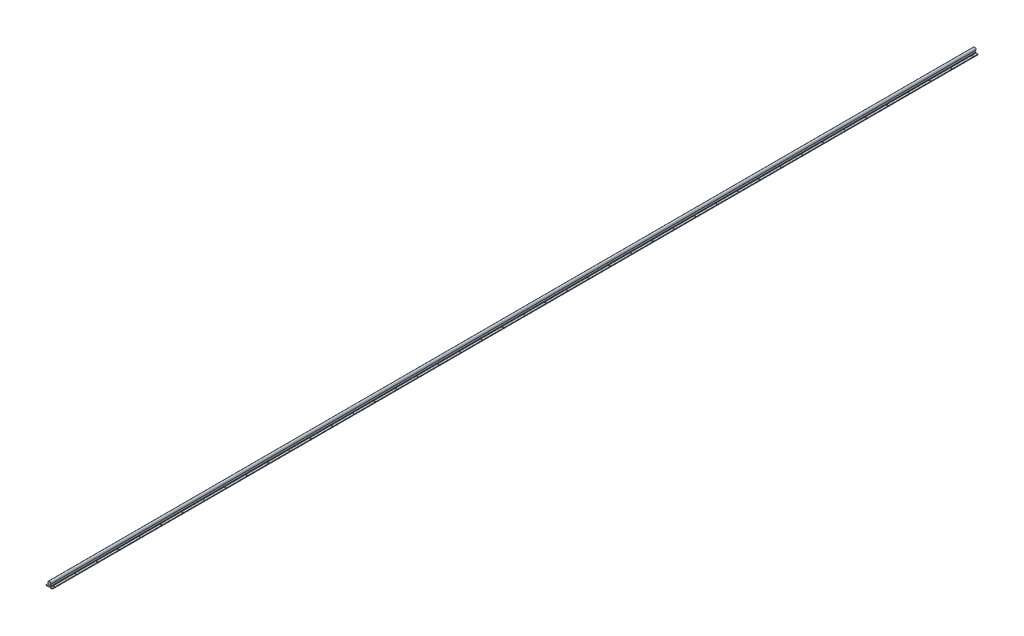
from build123d import *

# Parameters (mm, degrees)
BOSS_EXTRUDE1_DEPTH        = 6500
SKETCH5_R                  = 2.75
CUT_EXTRUDE1_DEPTH         = 6501.117710473
LPATTERN1_COUNT            = 44
LPATTERN1_PITCH            = 150
LPATTERN1_COPY_1_SKETCH_R  = 2.75
LPATTERN1_COPY_1_DEPTH     = 6501.117710473
LPATTERN1_COPY_2_SKETCH_R  = 2.75
LPATTERN1_COPY_2_DEPTH     = 6501.117710473
LPATTERN1_COPY_3_SKETCH_R  = 2.75
LPATTERN1_COPY_3_DEPTH     = 6501.117710473
LPATTERN1_COPY_4_SKETCH_R  = 2.75
LPATTERN1_COPY_4_DEPTH     = 6501.117710473
LPATTERN1_COPY_5_SKETCH_R  = 2.75
LPATTERN1_COPY_5_DEPTH     = 6501.117710473
LPATTERN1_COPY_6_SKETCH_R  = 2.75
LPATTERN1_COPY_6_DEPTH     = 6501.117710473
LPATTERN1_COPY_7_SKETCH_R  = 2.75
LPATTERN1_COPY_7_DEPTH     = 6501.117710473
LPATTERN1_COPY_8_SKETCH_R  = 2.75
LPATTERN1_COPY_8_DEPTH     = 6501.117710473
LPATTERN1_COPY_9_SKETCH_R  = 2.75
LPATTERN1_COPY_9_DEPTH     = 6501.117710473
LPATTERN1_COPY_10_SKETCH_R = 2.75
LPATTERN1_COPY_10_DEPTH    = 6501.117710473
LPATTERN1_COPY_11_SKETCH_R = 2.75
LPATTERN1_COPY_11_DEPTH    = 6501.117710473
LPATTERN1_COPY_12_SKETCH_R = 2.75
LPATTERN1_COPY_12_DEPTH    = 6501.117710473
LPATTERN1_COPY_13_SKETCH_R = 2.75
LPATTERN1_COPY_13_DEPTH    = 6501.117710473
LPATTERN1_COPY_14_SKETCH_R = 2.75
LPATTERN1_COPY_14_DEPTH    = 6501.117710473
LPATTERN1_COPY_15_SKETCH_R = 2.75
LPATTERN1_COPY_15_DEPTH    = 6501.117710473
LPATTERN1_COPY_16_SKETCH_R = 2.75
LPATTERN1_COPY_16_DEPTH    = 6501.117710473
LPATTERN1_COPY_17_SKETCH_R = 2.75
LPATTERN1_COPY_17_DEPTH    = 6501.117710473
LPATTERN1_COPY_18_SKETCH_R = 2.75
LPATTERN1_COPY_18_DEPTH    = 6501.117710473
LPATTERN1_COPY_19_SKETCH_R = 2.75
LPATTERN1_COPY_19_DEPTH    = 6501.117710473
LPATTERN1_COPY_20_SKETCH_R = 2.75
LPATTERN1_COPY_20_DEPTH    = 6501.117710473
LPATTERN1_COPY_21_SKETCH_R = 2.75
LPATTERN1_COPY_21_DEPTH    = 6501.117710473
LPATTERN1_COPY_22_SKETCH_R = 2.75
LPATTERN1_COPY_22_DEPTH    = 6501.117710473
LPATTERN1_COPY_23_SKETCH_R = 2.75
LPATTERN1_COPY_23_DEPTH    = 6501.117710473
LPATTERN1_COPY_24_SKETCH_R = 2.75
LPATTERN1_COPY_24_DEPTH    = 6501.117710473
LPATTERN1_COPY_25_SKETCH_R = 2.75
LPATTERN1_COPY_25_DEPTH    = 6501.117710473
LPATTERN1_COPY_26_SKETCH_R = 2.75
LPATTERN1_COPY_26_DEPTH    = 6501.117710473
LPATTERN1_COPY_27_SKETCH_R = 2.75
LPATTERN1_COPY_27_DEPTH    = 6501.117710473
LPATTERN1_COPY_28_SKETCH_R = 2.75
LPATTERN1_COPY_28_DEPTH    = 6501.117710473
LPATTERN1_COPY_29_SKETCH_R = 2.75
LPATTERN1_COPY_29_DEPTH    = 6501.117710473
LPATTERN1_COPY_30_SKETCH_R = 2.75
LPATTERN1_COPY_30_DEPTH    = 6501.117710473
LPATTERN1_COPY_31_SKETCH_R = 2.75
LPATTERN1_COPY_31_DEPTH    = 6501.117710473
LPATTERN1_COPY_32_SKETCH_R = 2.75
LPATTERN1_COPY_32_DEPTH    = 6501.117710473
LPATTERN1_COPY_33_SKETCH_R = 2.75
LPATTERN1_COPY_33_DEPTH    = 6501.117710473
LPATTERN1_COPY_34_SKETCH_R = 2.75
LPATTERN1_COPY_34_DEPTH    = 6501.117710473
LPATTERN1_COPY_35_SKETCH_R = 2.75
LPATTERN1_COPY_35_DEPTH    = 6501.117710473
LPATTERN1_COPY_36_SKETCH_R = 2.75
LPATTERN1_COPY_36_DEPTH    = 6501.117710473
LPATTERN1_COPY_37_SKETCH_R = 2.75
LPATTERN1_COPY_37_DEPTH    = 6501.117710473
LPATTERN1_COPY_38_SKETCH_R = 2.75
LPATTERN1_COPY_38_DEPTH    = 6501.117710473
LPATTERN1_COPY_39_SKETCH_R = 2.75
LPATTERN1_COPY_39_DEPTH    = 6501.117710473
LPATTERN1_COPY_40_SKETCH_R = 2.75
LPATTERN1_COPY_40_DEPTH    = 6501.117710473
LPATTERN1_COPY_41_SKETCH_R = 2.75
LPATTERN1_COPY_41_DEPTH    = 6501.117710473
LPATTERN1_COPY_42_SKETCH_R = 2.75
LPATTERN1_COPY_42_DEPTH    = 6501.117710473
LPATTERN1_COPY_43_SKETCH_R = 2.75
LPATTERN1_COPY_43_DEPTH    = 6501.117710473
CHAMFER1_SIZE              = 1


with BuildPart() as part:
    # Sketch3 → Boss-Extrude1 (new body)
    with BuildSketch(Plane.XY):
        with BuildLine():
            Line((-5.5, -20.5), (5.5, -20.5))
            Line((5.5, -20.5), (5.5, -27))
            Line((5.5, -27), (22.5, -27))
            Line((22.5, -27), (22.5, -22))
            Line((22.5, -22), (9.5, -22))
            Line((9.5, -22), (9.5, -17))
            Line((9.5, -17), (8.445597073, -17))
            Line((8.445597073, -17), (4, -9.3))
            Line((4, -9.3), (4, -9.16515139))
            ThreePointArc((4, -9.16515139), (0, 10), (-4, -9.16515139))
            Line((-4, -9.16515139), (-4, -9.3))
            Line((-4, -9.3), (-8.445597073, -17))
            Line((-8.445597073, -17), (-9.5, -17))
            Line((-9.5, -17), (-9.5, -22))
            Line((-9.5, -22), (-22.5, -22))
            Line((-22.5, -22), (-22.5, -27))
            Line((-22.5, -27), (-5.5, -27))
            Line((-5.5, -27), (-5.5, -20.5))
        make_face()
    extrude(amount=-BOSS_EXTRUDE1_DEPTH)

    # Sketch4 → Cut-Revolve1 (revolve, cut)
    with BuildSketch(Plane(origin=(0, 0, 0), x_dir=(0, 0, -1), z_dir=(1, 0, 0)), mode=Mode.PRIVATE) as cut_revolve1_sk:
        Polygon((22.805, 2.195), (20, 5), (20, -27), (23.3, -27), (23.3, -9.3), (22.805, -8.805), align=None)
    cut_revolve1 = revolve(cut_revolve1_sk.sketch.rotate(Axis((0, 5, -20), (0, -1, 0)), 180), axis=Axis((0, 5, -20), (0, -1, 0)), mode=Mode.SUBTRACT)

    # Sketch5 → Cut-Extrude1 (cut, through all)
    with BuildSketch(Plane(origin=(0, -22, 0), x_dir=(1, 0, 0), z_dir=(0, 1, 0))):
        with Locations(Location((15, 20, 0), (0, 0, 270))):
            Circle(SKETCH5_R)
    cut_extrude1 = extrude(amount=-CUT_EXTRUDE1_DEPTH, mode=Mode.SUBTRACT)

    # Mirror1: Cut-Extrude1 across plane
    add(cut_extrude1.mirror(Plane(origin=(0, 0, 0), x_dir=(0, 0, 1), z_dir=(1, 0, 0))), mode=Mode.SUBTRACT)

    # LPattern1: Cut-Revolve1, Cut-Extrude1 ×44
    with Locations(*[(0, 0, -i * LPATTERN1_PITCH) for i in range(1, LPATTERN1_COUNT)]):
        add(cut_revolve1, mode=Mode.SUBTRACT)
        add(cut_extrude1, mode=Mode.SUBTRACT)

    # LPattern1 copy 1 sketch → LPattern1 copy 1 (cut, through all)
    with BuildSketch(Plane(origin=(0, -22, -150), x_dir=(-1, 0, 0), z_dir=(0, 1, 0))):
        with Locations((15, -20)):
            Circle(LPATTERN1_COPY_1_SKETCH_R)
    extrude(amount=-LPATTERN1_COPY_1_DEPTH, mode=Mode.SUBTRACT)

    # LPattern1 copy 2 sketch → LPattern1 copy 2 (cut, through all)
    with BuildSketch(Plane(origin=(0, -22, -300), x_dir=(-1, 0, 0), z_dir=(0, 1, 0))):
        with Locations((15, -20)):
            Circle(LPATTERN1_COPY_2_SKETCH_R)
    extrude(amount=-LPATTERN1_COPY_2_DEPTH, mode=Mode.SUBTRACT)

    # LPattern1 copy 3 sketch → LPattern1 copy 3 (cut, through all)
    with BuildSketch(Plane(origin=(0, -22, -450), x_dir=(-1, 0, 0), z_dir=(0, 1, 0))):
        with Locations((15, -20)):
            Circle(LPATTERN1_COPY_3_SKETCH_R)
    extrude(amount=-LPATTERN1_COPY_3_DEPTH, mode=Mode.SUBTRACT)

    # LPattern1 copy 4 sketch → LPattern1 copy 4 (cut, through all)
    with BuildSketch(Plane(origin=(0, -22, -600), x_dir=(-1, 0, 0), z_dir=(0, 1, 0))):
        with Locations((15, -20)):
            Circle(LPATTERN1_COPY_4_SKETCH_R)
    extrude(amount=-LPATTERN1_COPY_4_DEPTH, mode=Mode.SUBTRACT)

    # LPattern1 copy 5 sketch → LPattern1 copy 5 (cut, through all)
    with BuildSketch(Plane(origin=(0, -22, -750), x_dir=(-1, 0, 0), z_dir=(0, 1, 0))):
        with Locations((15, -20)):
            Circle(LPATTERN1_COPY_5_SKETCH_R)
    extrude(amount=-LPATTERN1_COPY_5_DEPTH, mode=Mode.SUBTRACT)

    # LPattern1 copy 6 sketch → LPattern1 copy 6 (cut, through all)
    with BuildSketch(Plane(origin=(0, -22, -900), x_dir=(-1, 0, 0), z_dir=(0, 1, 0))):
        with Locations((15, -20)):
            Circle(LPATTERN1_COPY_6_SKETCH_R)
    extrude(amount=-LPATTERN1_COPY_6_DEPTH, mode=Mode.SUBTRACT)

    # LPattern1 copy 7 sketch → LPattern1 copy 7 (cut, through all)
    with BuildSketch(Plane(origin=(0, -22, -1050), x_dir=(-1, 0, 0), z_dir=(0, 1, 0))):
        with Locations((15, -20)):
            Circle(LPATTERN1_COPY_7_SKETCH_R)
    extrude(amount=-LPATTERN1_COPY_7_DEPTH, mode=Mode.SUBTRACT)

    # LPattern1 copy 8 sketch → LPattern1 copy 8 (cut, through all)
    with BuildSketch(Plane(origin=(0, -22, -1200), x_dir=(-1, 0, 0), z_dir=(0, 1, 0))):
        with Locations((15, -20)):
            Circle(LPATTERN1_COPY_8_SKETCH_R)
    extrude(amount=-LPATTERN1_COPY_8_DEPTH, mode=Mode.SUBTRACT)

    # LPattern1 copy 9 sketch → LPattern1 copy 9 (cut, through all)
    with BuildSketch(Plane(origin=(0, -22, -1350), x_dir=(-1, 0, 0), z_dir=(0, 1, 0))):
        with Locations((15, -20)):
            Circle(LPATTERN1_COPY_9_SKETCH_R)
    extrude(amount=-LPATTERN1_COPY_9_DEPTH, mode=Mode.SUBTRACT)

    # LPattern1 copy 10 sketch → LPattern1 copy 10 (cut, through all)
    with BuildSketch(Plane(origin=(0, -22, -1500), x_dir=(-1, 0, 0), z_dir=(0, 1, 0))):
        with Locations((15, -20)):
            Circle(LPATTERN1_COPY_10_SKETCH_R)
    extrude(amount=-LPATTERN1_COPY_10_DEPTH, mode=Mode.SUBTRACT)

    # LPattern1 copy 11 sketch → LPattern1 copy 11 (cut, through all)
    with BuildSketch(Plane(origin=(0, -22, -1650), x_dir=(-1, 0, 0), z_dir=(0, 1, 0))):
        with Locations((15, -20)):
            Circle(LPATTERN1_COPY_11_SKETCH_R)
    extrude(amount=-LPATTERN1_COPY_11_DEPTH, mode=Mode.SUBTRACT)

    # LPattern1 copy 12 sketch → LPattern1 copy 12 (cut, through all)
    with BuildSketch(Plane(origin=(0, -22, -1800), x_dir=(-1, 0, 0), z_dir=(0, 1, 0))):
        with Locations((15, -20)):
            Circle(LPATTERN1_COPY_12_SKETCH_R)
    extrude(amount=-LPATTERN1_COPY_12_DEPTH, mode=Mode.SUBTRACT)

    # LPattern1 copy 13 sketch → LPattern1 copy 13 (cut, through all)
    with BuildSketch(Plane(origin=(0, -22, -1950), x_dir=(-1, 0, 0), z_dir=(0, 1, 0))):
        with Locations((15, -20)):
            Circle(LPATTERN1_COPY_13_SKETCH_R)
    extrude(amount=-LPATTERN1_COPY_13_DEPTH, mode=Mode.SUBTRACT)

    # LPattern1 copy 14 sketch → LPattern1 copy 14 (cut, through all)
    with BuildSketch(Plane(origin=(0, -22, -2100), x_dir=(-1, 0, 0), z_dir=(0, 1, 0))):
        with Locations((15, -20)):
            Circle(LPATTERN1_COPY_14_SKETCH_R)
    extrude(amount=-LPATTERN1_COPY_14_DEPTH, mode=Mode.SUBTRACT)

    # LPattern1 copy 15 sketch → LPattern1 copy 15 (cut, through all)
    with BuildSketch(Plane(origin=(0, -22, -2250), x_dir=(-1, 0, 0), z_dir=(0, 1, 0))):
        with Locations((15, -20)):
            Circle(LPATTERN1_COPY_15_SKETCH_R)
    extrude(amount=-LPATTERN1_COPY_15_DEPTH, mode=Mode.SUBTRACT)

    # LPattern1 copy 16 sketch → LPattern1 copy 16 (cut, through all)
    with BuildSketch(Plane(origin=(0, -22, -2400), x_dir=(-1, 0, 0), z_dir=(0, 1, 0))):
        with Locations((15, -20)):
            Circle(LPATTERN1_COPY_16_SKETCH_R)
    extrude(amount=-LPATTERN1_COPY_16_DEPTH, mode=Mode.SUBTRACT)

    # LPattern1 copy 17 sketch → LPattern1 copy 17 (cut, through all)
    with BuildSketch(Plane(origin=(0, -22, -2550), x_dir=(-1, 0, 0), z_dir=(0, 1, 0))):
        with Locations((15, -20)):
            Circle(LPATTERN1_COPY_17_SKETCH_R)
    extrude(amount=-LPATTERN1_COPY_17_DEPTH, mode=Mode.SUBTRACT)

    # LPattern1 copy 18 sketch → LPattern1 copy 18 (cut, through all)
    with BuildSketch(Plane(origin=(0, -22, -2700), x_dir=(-1, 0, 0), z_dir=(0, 1, 0))):
        with Locations((15, -20)):
            Circle(LPATTERN1_COPY_18_SKETCH_R)
    extrude(amount=-LPATTERN1_COPY_18_DEPTH, mode=Mode.SUBTRACT)

    # LPattern1 copy 19 sketch → LPattern1 copy 19 (cut, through all)
    with BuildSketch(Plane(origin=(0, -22, -2850), x_dir=(-1, 0, 0), z_dir=(0, 1, 0))):
        with Locations((15, -20)):
            Circle(LPATTERN1_COPY_19_SKETCH_R)
    extrude(amount=-LPATTERN1_COPY_19_DEPTH, mode=Mode.SUBTRACT)

    # LPattern1 copy 20 sketch → LPattern1 copy 20 (cut, through all)
    with BuildSketch(Plane(origin=(0, -22, -3000), x_dir=(-1, 0, 0), z_dir=(0, 1, 0))):
        with Locations((15, -20)):
            Circle(LPATTERN1_COPY_20_SKETCH_R)
    extrude(amount=-LPATTERN1_COPY_20_DEPTH, mode=Mode.SUBTRACT)

    # LPattern1 copy 21 sketch → LPattern1 copy 21 (cut, through all)
    with BuildSketch(Plane(origin=(0, -22, -3150), x_dir=(-1, 0, 0), z_dir=(0, 1, 0))):
        with Locations((15, -20)):
            Circle(LPATTERN1_COPY_21_SKETCH_R)
    extrude(amount=-LPATTERN1_COPY_21_DEPTH, mode=Mode.SUBTRACT)

    # LPattern1 copy 22 sketch → LPattern1 copy 22 (cut, through all)
    with BuildSketch(Plane(origin=(0, -22, -3300), x_dir=(-1, 0, 0), z_dir=(0, 1, 0))):
        with Locations((15, -20)):
            Circle(LPATTERN1_COPY_22_SKETCH_R)
    extrude(amount=-LPATTERN1_COPY_22_DEPTH, mode=Mode.SUBTRACT)

    # LPattern1 copy 23 sketch → LPattern1 copy 23 (cut, through all)
    with BuildSketch(Plane(origin=(0, -22, -3450), x_dir=(-1, 0, 0), z_dir=(0, 1, 0))):
        with Locations((15, -20)):
            Circle(LPATTERN1_COPY_23_SKETCH_R)
    extrude(amount=-LPATTERN1_COPY_23_DEPTH, mode=Mode.SUBTRACT)

    # LPattern1 copy 24 sketch → LPattern1 copy 24 (cut, through all)
    with BuildSketch(Plane(origin=(0, -22, -3600), x_dir=(-1, 0, 0), z_dir=(0, 1, 0))):
        with Locations((15, -20)):
            Circle(LPATTERN1_COPY_24_SKETCH_R)
    extrude(amount=-LPATTERN1_COPY_24_DEPTH, mode=Mode.SUBTRACT)

    # LPattern1 copy 25 sketch → LPattern1 copy 25 (cut, through all)
    with BuildSketch(Plane(origin=(0, -22, -3750), x_dir=(-1, 0, 0), z_dir=(0, 1, 0))):
        with Locations((15, -20)):
            Circle(LPATTERN1_COPY_25_SKETCH_R)
    extrude(amount=-LPATTERN1_COPY_25_DEPTH, mode=Mode.SUBTRACT)

    # LPattern1 copy 26 sketch → LPattern1 copy 26 (cut, through all)
    with BuildSketch(Plane(origin=(0, -22, -3900), x_dir=(-1, 0, 0), z_dir=(0, 1, 0))):
        with Locations((15, -20)):
            Circle(LPATTERN1_COPY_26_SKETCH_R)
    extrude(amount=-LPATTERN1_COPY_26_DEPTH, mode=Mode.SUBTRACT)

    # LPattern1 copy 27 sketch → LPattern1 copy 27 (cut, through all)
    with BuildSketch(Plane(origin=(0, -22, -4050), x_dir=(-1, 0, 0), z_dir=(0, 1, 0))):
        with Locations((15, -20)):
            Circle(LPATTERN1_COPY_27_SKETCH_R)
    extrude(amount=-LPATTERN1_COPY_27_DEPTH, mode=Mode.SUBTRACT)

    # LPattern1 copy 28 sketch → LPattern1 copy 28 (cut, through all)
    with BuildSketch(Plane(origin=(0, -22, -4200), x_dir=(-1, 0, 0), z_dir=(0, 1, 0))):
        with Locations((15, -20)):
            Circle(LPATTERN1_COPY_28_SKETCH_R)
    extrude(amount=-LPATTERN1_COPY_28_DEPTH, mode=Mode.SUBTRACT)

    # LPattern1 copy 29 sketch → LPattern1 copy 29 (cut, through all)
    with BuildSketch(Plane(origin=(0, -22, -4350), x_dir=(-1, 0, 0), z_dir=(0, 1, 0))):
        with Locations((15, -20)):
            Circle(LPATTERN1_COPY_29_SKETCH_R)
    extrude(amount=-LPATTERN1_COPY_29_DEPTH, mode=Mode.SUBTRACT)

    # LPattern1 copy 30 sketch → LPattern1 copy 30 (cut, through all)
    with BuildSketch(Plane(origin=(0, -22, -4500), x_dir=(-1, 0, 0), z_dir=(0, 1, 0))):
        with Locations((15, -20)):
            Circle(LPATTERN1_COPY_30_SKETCH_R)
    extrude(amount=-LPATTERN1_COPY_30_DEPTH, mode=Mode.SUBTRACT)

    # LPattern1 copy 31 sketch → LPattern1 copy 31 (cut, through all)
    with BuildSketch(Plane(origin=(0, -22, -4650), x_dir=(-1, 0, 0), z_dir=(0, 1, 0))):
        with Locations((15, -20)):
            Circle(LPATTERN1_COPY_31_SKETCH_R)
    extrude(amount=-LPATTERN1_COPY_31_DEPTH, mode=Mode.SUBTRACT)

    # LPattern1 copy 32 sketch → LPattern1 copy 32 (cut, through all)
    with BuildSketch(Plane(origin=(0, -22, -4800), x_dir=(-1, 0, 0), z_dir=(0, 1, 0))):
        with Locations((15, -20)):
            Circle(LPATTERN1_COPY_32_SKETCH_R)
    extrude(amount=-LPATTERN1_COPY_32_DEPTH, mode=Mode.SUBTRACT)

    # LPattern1 copy 33 sketch → LPattern1 copy 33 (cut, through all)
    with BuildSketch(Plane(origin=(0, -22, -4950), x_dir=(-1, 0, 0), z_dir=(0, 1, 0))):
        with Locations((15, -20)):
            Circle(LPATTERN1_COPY_33_SKETCH_R)
    extrude(amount=-LPATTERN1_COPY_33_DEPTH, mode=Mode.SUBTRACT)

    # LPattern1 copy 34 sketch → LPattern1 copy 34 (cut, through all)
    with BuildSketch(Plane(origin=(0, -22, -5100), x_dir=(-1, 0, 0), z_dir=(0, 1, 0))):
        with Locations((15, -20)):
            Circle(LPATTERN1_COPY_34_SKETCH_R)
    extrude(amount=-LPATTERN1_COPY_34_DEPTH, mode=Mode.SUBTRACT)

    # LPattern1 copy 35 sketch → LPattern1 copy 35 (cut, through all)
    with BuildSketch(Plane(origin=(0, -22, -5250), x_dir=(-1, 0, 0), z_dir=(0, 1, 0))):
        with Locations((15, -20)):
            Circle(LPATTERN1_COPY_35_SKETCH_R)
    extrude(amount=-LPATTERN1_COPY_35_DEPTH, mode=Mode.SUBTRACT)

    # LPattern1 copy 36 sketch → LPattern1 copy 36 (cut, through all)
    with BuildSketch(Plane(origin=(0, -22, -5400), x_dir=(-1, 0, 0), z_dir=(0, 1, 0))):
        with Locations((15, -20)):
            Circle(LPATTERN1_COPY_36_SKETCH_R)
    extrude(amount=-LPATTERN1_COPY_36_DEPTH, mode=Mode.SUBTRACT)

    # LPattern1 copy 37 sketch → LPattern1 copy 37 (cut, through all)
    with BuildSketch(Plane(origin=(0, -22, -5550), x_dir=(-1, 0, 0), z_dir=(0, 1, 0))):
        with Locations((15, -20)):
            Circle(LPATTERN1_COPY_37_SKETCH_R)
    extrude(amount=-LPATTERN1_COPY_37_DEPTH, mode=Mode.SUBTRACT)

    # LPattern1 copy 38 sketch → LPattern1 copy 38 (cut, through all)
    with BuildSketch(Plane(origin=(0, -22, -5700), x_dir=(-1, 0, 0), z_dir=(0, 1, 0))):
        with Locations((15, -20)):
            Circle(LPATTERN1_COPY_38_SKETCH_R)
    extrude(amount=-LPATTERN1_COPY_38_DEPTH, mode=Mode.SUBTRACT)

    # LPattern1 copy 39 sketch → LPattern1 copy 39 (cut, through all)
    with BuildSketch(Plane(origin=(0, -22, -5850), x_dir=(-1, 0, 0), z_dir=(0, 1, 0))):
        with Locations((15, -20)):
            Circle(LPATTERN1_COPY_39_SKETCH_R)
    extrude(amount=-LPATTERN1_COPY_39_DEPTH, mode=Mode.SUBTRACT)

    # LPattern1 copy 40 sketch → LPattern1 copy 40 (cut, through all)
    with BuildSketch(Plane(origin=(0, -22, -6000), x_dir=(-1, 0, 0), z_dir=(0, 1, 0))):
        with Locations((15, -20)):
            Circle(LPATTERN1_COPY_40_SKETCH_R)
    extrude(amount=-LPATTERN1_COPY_40_DEPTH, mode=Mode.SUBTRACT)

    # LPattern1 copy 41 sketch → LPattern1 copy 41 (cut, through all)
    with BuildSketch(Plane(origin=(0, -22, -6150), x_dir=(-1, 0, 0), z_dir=(0, 1, 0))):
        with Locations((15, -20)):
            Circle(LPATTERN1_COPY_41_SKETCH_R)
    extrude(amount=-LPATTERN1_COPY_41_DEPTH, mode=Mode.SUBTRACT)

    # LPattern1 copy 42 sketch → LPattern1 copy 42 (cut, through all)
    with BuildSketch(Plane(origin=(0, -22, -6300), x_dir=(-1, 0, 0), z_dir=(0, 1, 0))):
        with Locations((15, -20)):
            Circle(LPATTERN1_COPY_42_SKETCH_R)
    extrude(amount=-LPATTERN1_COPY_42_DEPTH, mode=Mode.SUBTRACT)

    # LPattern1 copy 43 sketch → LPattern1 copy 43 (cut, through all)
    with BuildSketch(Plane(origin=(0, -22, -6450), x_dir=(-1, 0, 0), z_dir=(0, 1, 0))):
        with Locations((15, -20)):
            Circle(LPATTERN1_COPY_43_SKETCH_R)
    extrude(amount=-LPATTERN1_COPY_43_DEPTH, mode=Mode.SUBTRACT)

    # Chamfer1
    chamfer1_edges = [part.edges().sort_by_distance(p)[0] for p in [
        (0, 10, 0),
        (0, 10, -6500),
    ]]
    chamfer(chamfer1_edges, length=CHAMFER1_SIZE)


solid = part.part
